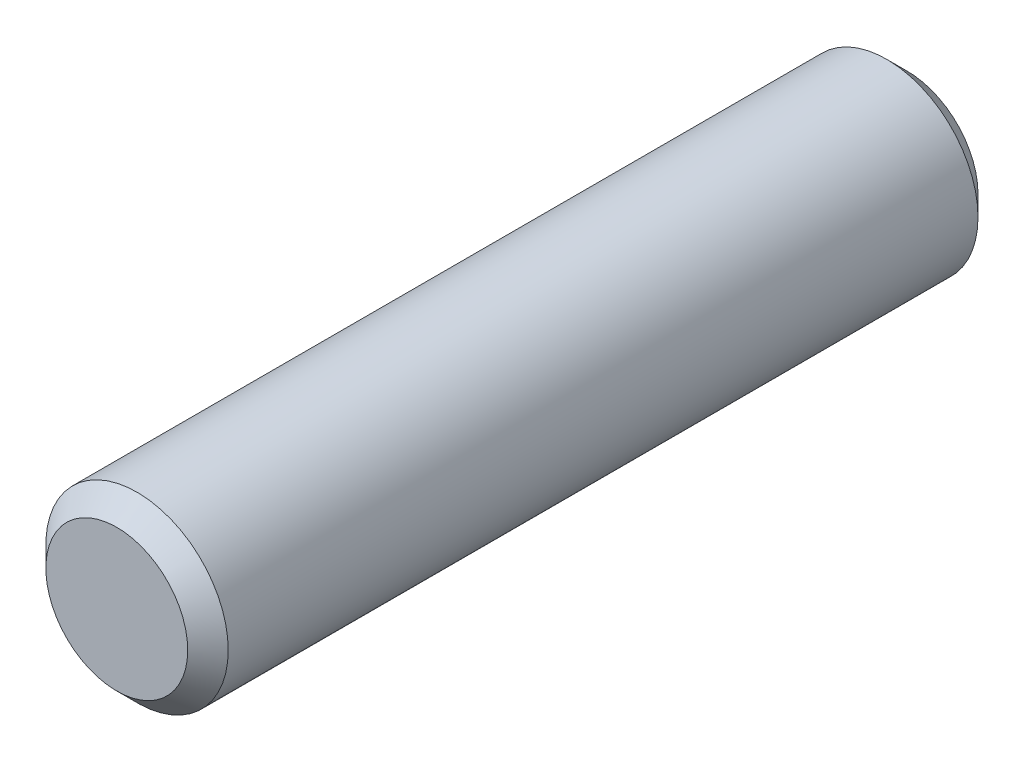
SolidWorks part; units mm, degrees
ref_plane "Front Plane" through (0, 0, 0) normal (0, 0, 1) x (1, 0, 0)
ref_plane "Top Plane" through (0, 0, 0) normal (0, 1, 0) x (1, 0, 0)
ref_plane "Right Plane" through (0, 0, 0) normal (1, 0, 0) x (0, 0, -1)
sketch "Sketch1" plane through (0, 0, 0) normal (0, 0, 1) x (1, 0, 0)
  circle A0 centre (0, 0) radius 4.5
  dimension "D1" = 9
extrude "Boss-Extrude1" add sketch "Sketch1" along normal blind 39
chamfer "Chamfer1" distance 1 angle 45 2 edges at (4.5, 0, 0) (4.5, 0, 39)
